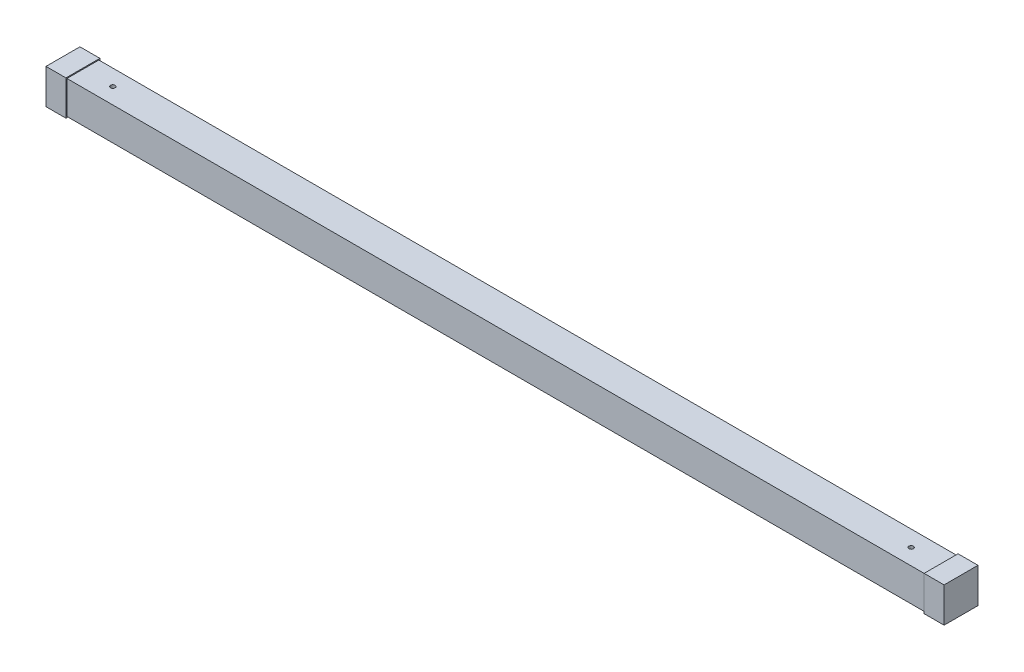
from build123d import *

# Parameters (mm, degrees)
SKETCH_1_W                  = 900
SKETCH_1_H                  = 33
EXTRUDE_1_DEPTH             = 16
SKETCH_2_W                  = 34
SKETCH_2_H                  = 35
EXTRUDE_2_DEPTH             = 20
HOLE_WIZARD_4_5_4_5_1_D     = 4.5
HOLE_WIZARD_4_5_4_5_1_DEPTH = 10
HOLE_WIZARD_4_5_4_5_1_TIP   = 1.351936393


with BuildPart() as part:
    # 草图1 → 凸台-拉伸1 (new, symmetric)
    with BuildSketch(Plane.XY):
        Rectangle(SKETCH_1_W, SKETCH_1_H)
    extrude(amount=EXTRUDE_1_DEPTH, both=True)

    # 草图2 → 凸台-拉伸2 (add)
    with BuildSketch(Plane(origin=(450, 0, 0), x_dir=(0, 0, -1), z_dir=(1, 0, 0))):
        Rectangle(SKETCH_2_W, SKETCH_2_H)
    extrude_2 = extrude(amount=-EXTRUDE_2_DEPTH)

    # 镜向2: 凸台-拉伸2 across plane
    add(extrude_2.mirror(Plane(origin=(0, 0, 0), x_dir=(0, 0, 1), z_dir=(1, 0, 0))))

    # Ø4.5 (4.5) 直径孔1
    with Locations(Plane(origin=(0, 16.5, 0), x_dir=(1, 0, 0), z_dir=(0, 1, 0))):
        with Locations((-400, 0), (400, 0)):
            Hole(HOLE_WIZARD_4_5_4_5_1_D / 2, depth=HOLE_WIZARD_4_5_4_5_1_DEPTH)
            with Locations((0, 0, -(HOLE_WIZARD_4_5_4_5_1_DEPTH + HOLE_WIZARD_4_5_4_5_1_TIP / 2))):  # 118° drill point
                Cone(0, HOLE_WIZARD_4_5_4_5_1_D / 2, HOLE_WIZARD_4_5_4_5_1_TIP, mode=Mode.SUBTRACT)


solid = part.part
